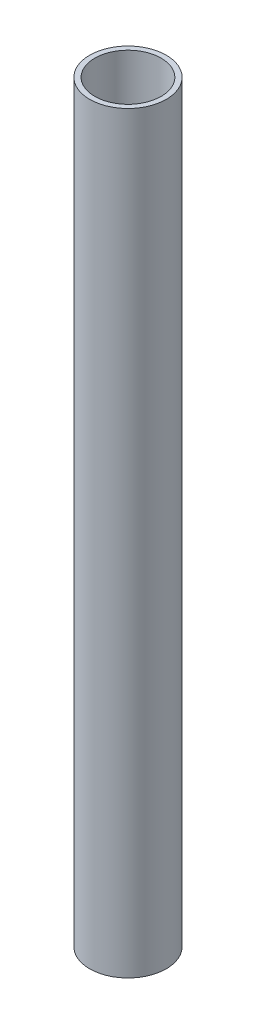
SolidWorks part; units mm, degrees
material "Q235B"
ref_plane "Front Plane" through (0, 0, 0) normal (0, 0, 1) x (1, 0, 0)
ref_plane "Top Plane" through (0, 0, 0) normal (0, 1, 0) x (1, 0, 0)
ref_plane "Right Plane" through (0, 0, 0) normal (1, 0, 0) x (0, 0, -1)
sketch "Sketch1" plane through (0, 0, 0) normal (0, 0, 1) x (1, 0, 0)
  line L0 (0, 0) -> (0, 590)
  dimension "D1" = 590
other "Gb/t 6728-2002 round tube 60 × 4(1)"
ref_plane "Plane1" through (0, 0, 0) normal (0, 1, 0) x (-1, 0, 0)
sketch "Sketch11" plane through (0, 0, 0) normal (0, 1, 0) x (-1, 0, 0)
  circle A0 centre (0, 0) radius 26
  circle A1 centre (0, 0) radius 30
  point P3 (0, 0)
  dimension "Out_dia" = 60
  dimension "D1" = 4
  dimension "D2" = 52
